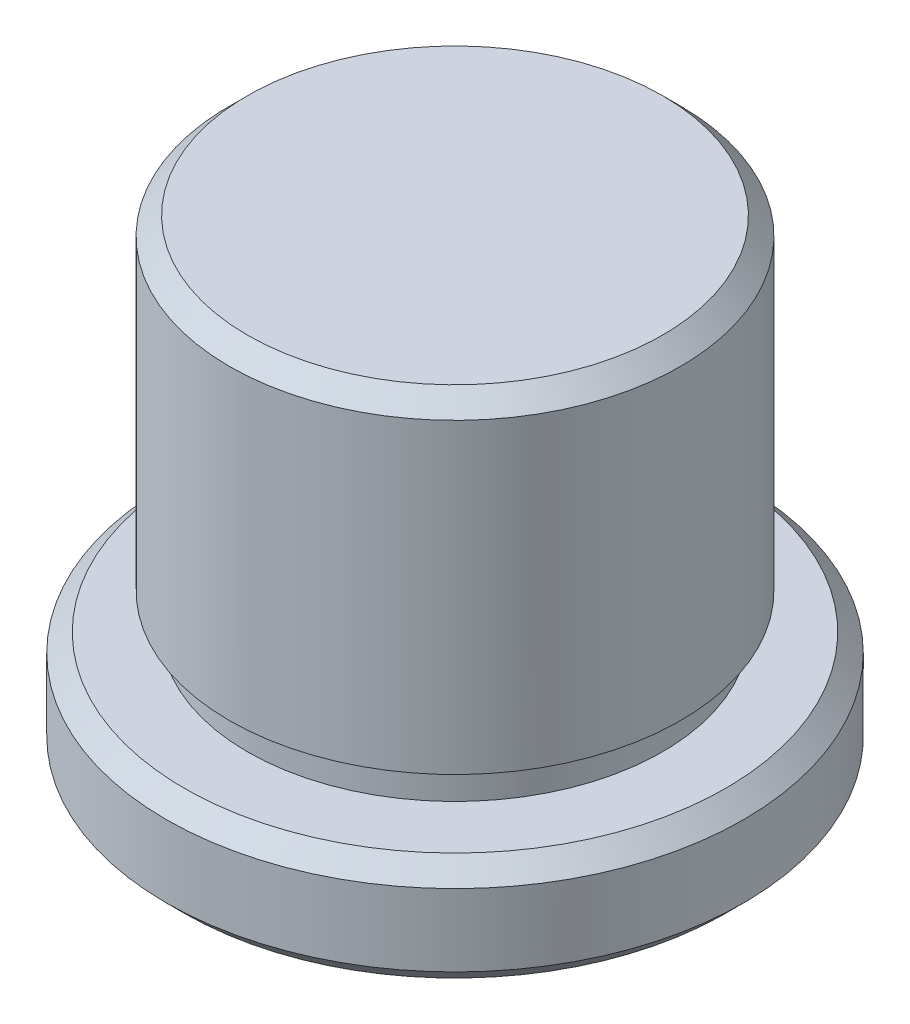
from build123d import *

# Parameters (mm, degrees)
CHAMFER1_SIZE = 0.5


with BuildPart() as part:
    # Sketch1 → Revolve1 (revolve)
    with BuildSketch(Plane.XY, mode=Mode.PRIVATE) as revolve1_sk:
        Polygon((74.023669398, -131.5), (74.023669398, -118.5), (80.273669398, -118.5), (80.273669398, -127.5), (79.773669398, -127.5), (79.773669398, -128.5), (82.023669398, -128.5), (82.023669398, -131.5), align=None)
    revolve(revolve1_sk.sketch.rotate(Axis((74.023669398, -118.5, 0), (0, -1, 0)), 90), axis=Axis((74.023669398, -118.5, 0), (0, -1, 0)))

    # Chamfer1
    chamfer1_edges = [part.edges().sort_by_distance(p)[0] for p in [
        (74.023669398, -131.5, -8),
        (74.023669398, -128.5, -8),
        (74.023669398, -118.5, -6.25),
    ]]
    chamfer(chamfer1_edges, length=CHAMFER1_SIZE)


solid = part.part
